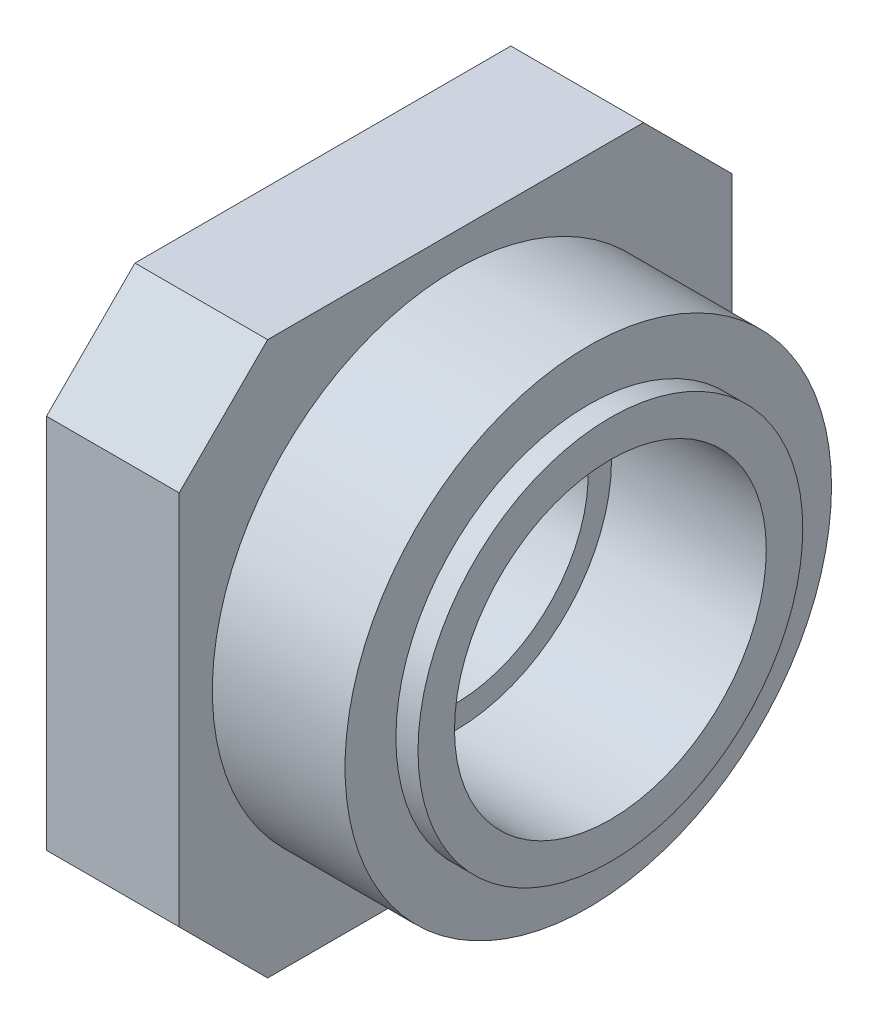
from build123d import *

# Parameters (mm, degrees)
SKETCH1_W              = 25
SKETCH1_H              = 25
BOSS_EXTRUDE1_DEPTH    = 3
M14_TAPPED_HOLE1_D     = 12
M14_TAPPED_HOLE1_DEPTH = 34
M14_TAPPED_HOLE1_TIP   = 3.605163714
SKETCH5_R              = 11
SKETCH5_R_2            = 7.05
BOSS_EXTRUDE2_DEPTH    = 7
CUT_EXTRUDE1_START     = -1
SKETCH6_R              = 11
SKETCH6_R_2            = 8.7
CUT_EXTRUDE1_DEPTH     = 1
CHAMFER1_SIZE          = 4


with BuildPart() as part:
    # Sketch1 → Boss-Extrude1 (new, symmetric)
    with BuildSketch(Plane(origin=(0, 0, 0), x_dir=(0, 0, -1), z_dir=(1, 0, 0))):
        Rectangle(SKETCH1_W, SKETCH1_H)
    extrude(amount=BOSS_EXTRUDE1_DEPTH, both=True)

    # M14 Tapped Hole1
    with Locations(Plane.ZY.offset(3)):
        with Locations((0, 0)):
            Hole(M14_TAPPED_HOLE1_D / 2, depth=M14_TAPPED_HOLE1_DEPTH)
            with Locations((0, 0, -(M14_TAPPED_HOLE1_DEPTH + M14_TAPPED_HOLE1_TIP / 2))):  # 118° drill point
                Cone(0, M14_TAPPED_HOLE1_D / 2, M14_TAPPED_HOLE1_TIP, mode=Mode.SUBTRACT)

    # Sketch5 → Boss-Extrude2 (add)
    with BuildSketch(Plane(origin=(3, 0, 0), x_dir=(0, 0, -1), z_dir=(1, 0, 0))):
        Circle(SKETCH5_R)
        Circle(SKETCH5_R_2, mode=Mode.SUBTRACT)
    extrude(amount=BOSS_EXTRUDE2_DEPTH)

    # Sketch6 → Cut-Extrude1 (cut)
    with BuildSketch(Plane(origin=(10, 0, 0), x_dir=(0, 0, -1), z_dir=(1, 0, 0)).offset(CUT_EXTRUDE1_START)):
        Circle(SKETCH6_R)
        Circle(SKETCH6_R_2, mode=Mode.SUBTRACT)
    extrude(amount=CUT_EXTRUDE1_DEPTH, mode=Mode.SUBTRACT)

    # Chamfer1
    chamfer1_edges = [part.edges().sort_by_distance(p)[0] for p in [
        (0, -12.5, -12.5),
        (0, -12.5, 12.5),
        (0, 12.5, 12.5),
        (0, 12.5, -12.5),
    ]]
    chamfer(chamfer1_edges, length=CHAMFER1_SIZE)


solid = part.part
